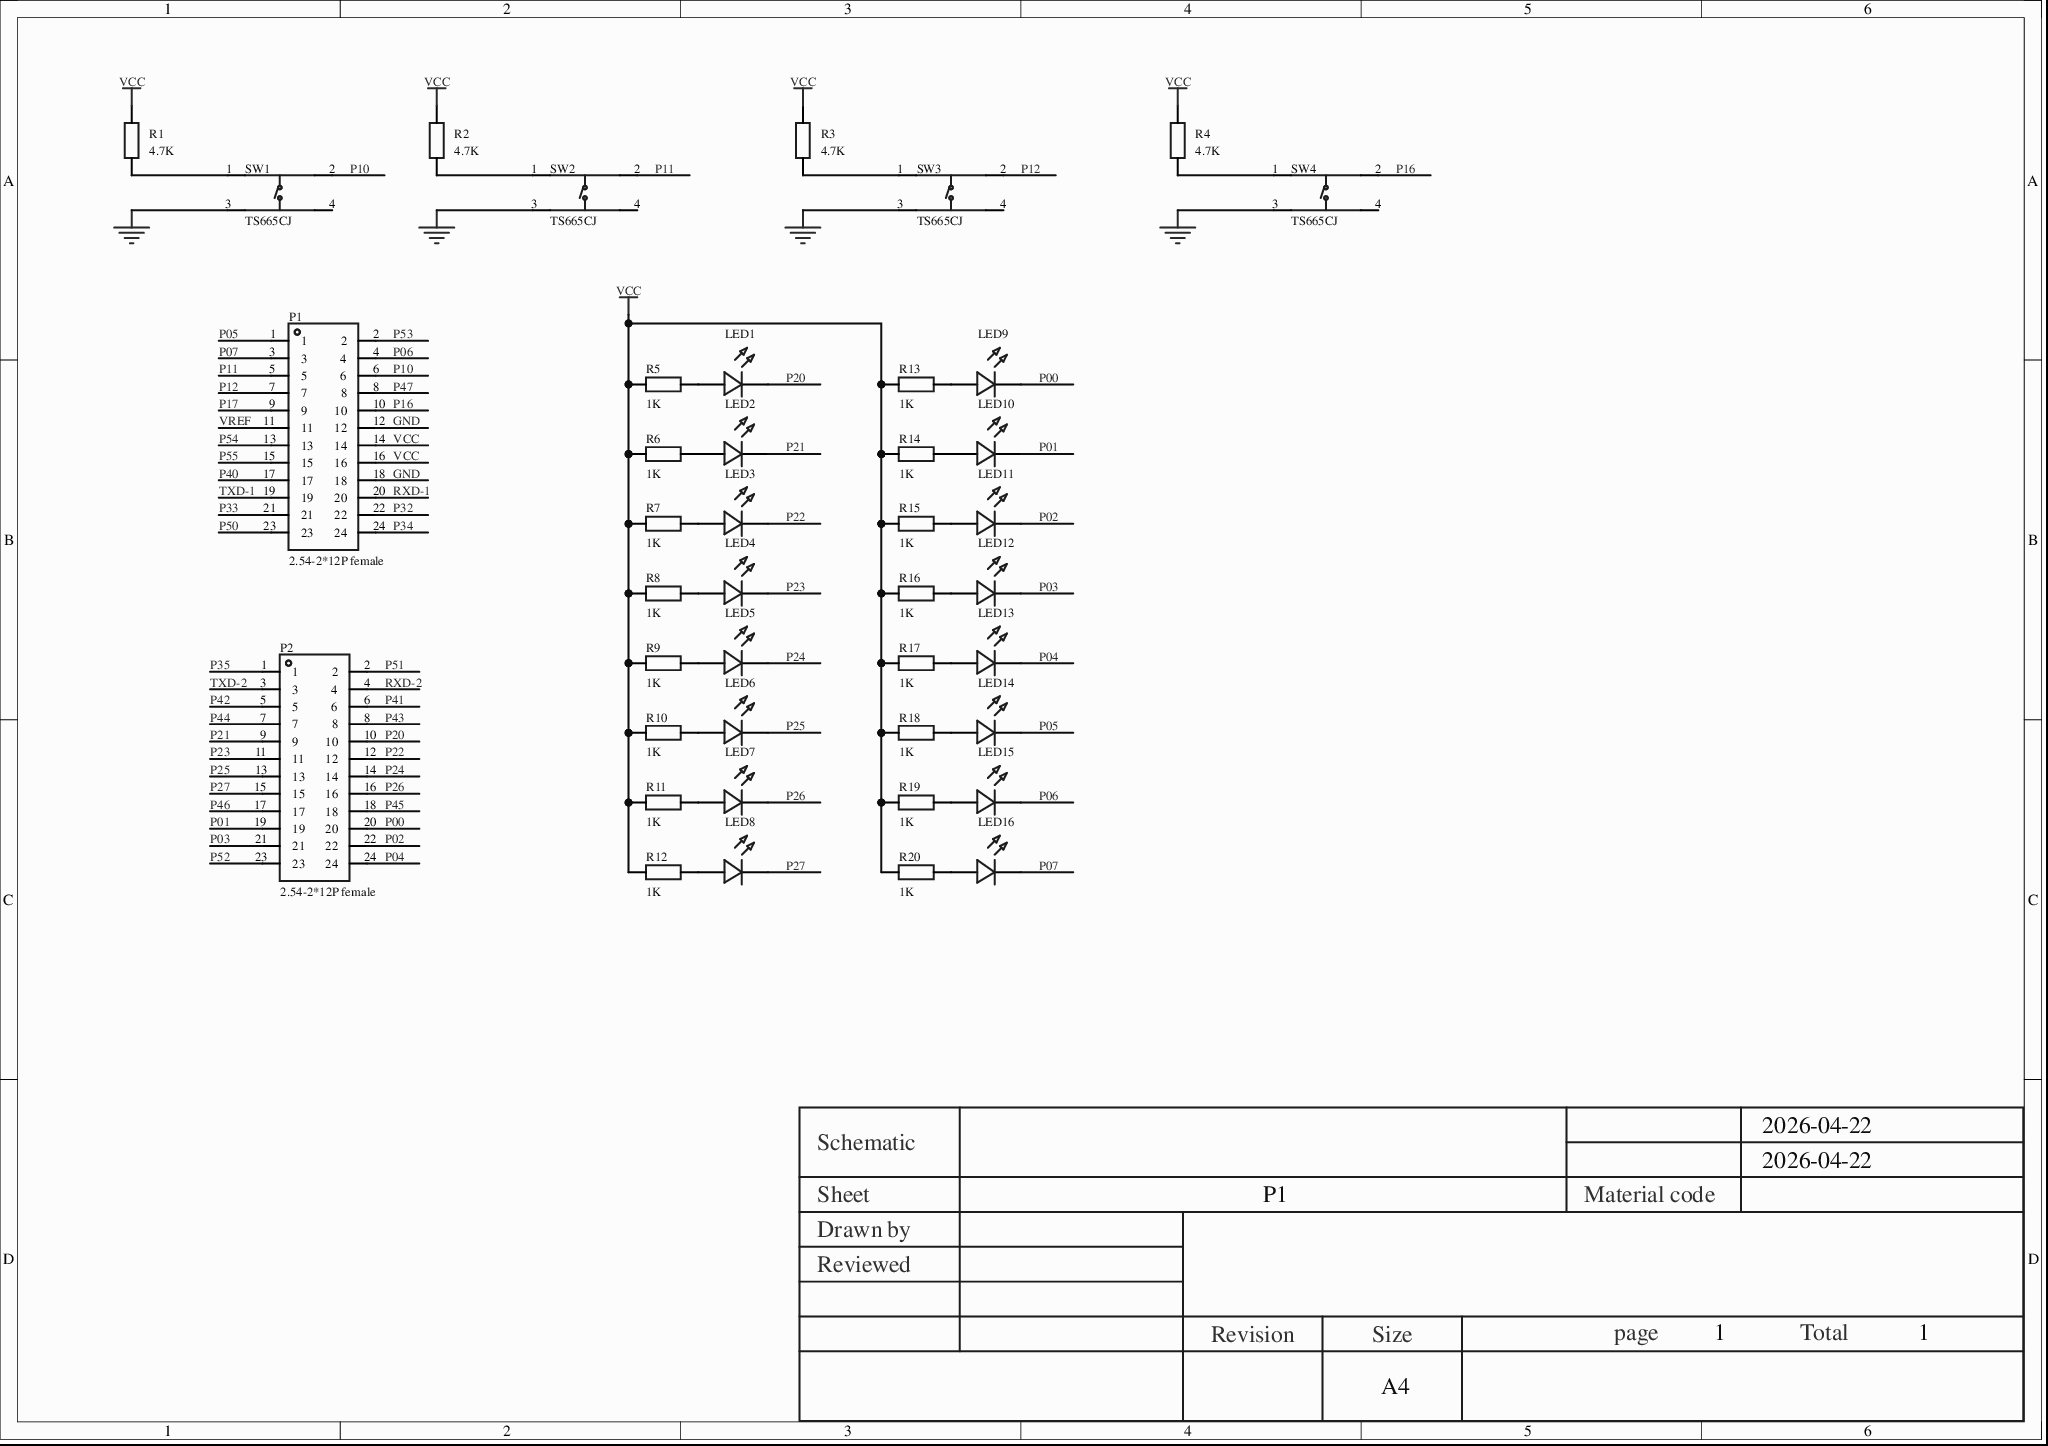
[diagram p0: MISC51818-3.schdoc]
# Altium project MISC51818-2.PrjPcb
1 sheet, 42 parts. Net scope: global (net labels, ports and power ports of the same name join across sheets).
Board file: MISC51818.pcbdoc

## Sheet MISC51818-3.schdoc
size 297 x 209 mm; Version: V1.0; @Project Name: MISC51818; @Page Count: 1; @Update Date: 2026-04-22; @Create Date: 2026-04-22; @Schematic Name: MISC51818; @Page No: 1; @Board Name: MISC51818; @Create Time: 22:35:28; @Update Time: 22:35:28

### Parts
LED1  (no value)  [LED-TH_L5.0-W5.0-P2.54_RED]
LED2  (no value)  [LED-TH_L5.0-W5.0-P2.54_RED]
LED3  (no value)  [LED-TH_L5.0-W5.0-P2.54_RED]
LED4  (no value)  [LED-TH_L5.0-W5.0-P2.54_RED]
LED5  (no value)  [LED-TH_L5.0-W5.0-P2.54_RED]
LED6  (no value)  [LED-TH_L5.0-W5.0-P2.54_RED]
LED7  (no value)  [LED-TH_L5.0-W5.0-P2.54_RED]
LED8  (no value)  [LED-TH_L5.0-W5.0-P2.54_RED]
LED9  (no value)  [LED-TH_L5.0-W5.0-P2.54_RED]
LED10  (no value)  [LED-TH_L5.0-W5.0-P2.54_RED]
LED11  (no value)  [LED-TH_L5.0-W5.0-P2.54_RED]
LED12  (no value)  [LED-TH_L5.0-W5.0-P2.54_RED]
LED13  (no value)  [LED-TH_L5.0-W5.0-P2.54_RED]
LED14  (no value)  [LED-TH_L5.0-W5.0-P2.54_RED]
LED15  (no value)  [LED-TH_L5.0-W5.0-P2.54_RED]
LED16  (no value)  [LED-TH_L5.0-W5.0-P2.54_RED]
P1  2.54-2*12P female  [HDR-TH_24P-P2.54-V-F-R2-C12-S2.54]
P2  2.54-2*12P female  [HDR-TH_24P-P2.54-V-F-R2-C12-S2.54]
R1  4.7K  [RES-TH_RES-TH_L6.5-W5.0-P2.50-D0.4-S2.00]
R2  4.7K  [RES-TH_RES-TH_L6.5-W5.0-P2.50-D0.4-S2.00]
R3  4.7K  [RES-TH_RES-TH_L6.5-W5.0-P2.50-D0.4-S2.00]
R4  4.7K  [RES-TH_RES-TH_L6.5-W5.0-P2.50-D0.4-S2.00]
R5  1K  [RES-TH_RES-TH_L6.5-W5.0-P2.50-D0.4-S2.00]
R6  1K  [RES-TH_RES-TH_L6.5-W5.0-P2.50-D0.4-S2.00]
R7  1K  [RES-TH_RES-TH_L6.5-W5.0-P2.50-D0.4-S2.00]
R8  1K  [RES-TH_RES-TH_L6.5-W5.0-P2.50-D0.4-S2.00]
R9  1K  [RES-TH_RES-TH_L6.5-W5.0-P2.50-D0.4-S2.00]
R10  1K  [RES-TH_RES-TH_L6.5-W5.0-P2.50-D0.4-S2.00]
R11  1K  [RES-TH_RES-TH_L6.5-W5.0-P2.50-D0.4-S2.00]
R12  1K  [RES-TH_RES-TH_L6.5-W5.0-P2.50-D0.4-S2.00]
R13  1K  [RES-TH_RES-TH_L6.5-W5.0-P2.50-D0.4-S2.00]
R14  1K  [RES-TH_RES-TH_L6.5-W5.0-P2.50-D0.4-S2.00]
R15  1K  [RES-TH_RES-TH_L6.5-W5.0-P2.50-D0.4-S2.00]
R16  1K  [RES-TH_RES-TH_L6.5-W5.0-P2.50-D0.4-S2.00]
R17  1K  [RES-TH_RES-TH_L6.5-W5.0-P2.50-D0.4-S2.00]
R18  1K  [RES-TH_RES-TH_L6.5-W5.0-P2.50-D0.4-S2.00]
R19  1K  [RES-TH_RES-TH_L6.5-W5.0-P2.50-D0.4-S2.00]
R20  1K  [RES-TH_RES-TH_L6.5-W5.0-P2.50-D0.4-S2.00]
SW1  TS665CJ  [SW-TH_4P-L6.0-W6.0-P4.50-LS6.5]
SW2  TS665CJ  [SW-TH_4P-L6.0-W6.0-P4.50-LS6.5]
SW3  TS665CJ  [SW-TH_4P-L6.0-W6.0-P4.50-LS6.5]
SW4  TS665CJ  [SW-TH_4P-L6.0-W6.0-P4.50-LS6.5]

### Nets
GND: P1.12 P1.18 SW1.3(C) SW2.3(C) SW3.3(C) SW4.3(C)
VCC: P1.14 P1.16 R1.2 R2.2 R3.2 R4.2 R5.1 R6.1 R7.1 R8.1 R9.1 R10.1 R11.1 R12.1 R13.1 R14.1 R15.1 R16.1 R17.1 R18.1 R19.1 R20.1
P00: LED9.1(C) P2.20
P01: LED10.1(C) P2.19
P02: LED11.1(C) P2.22
P03: LED12.1(C) P2.21
P04: LED13.1(C) P2.24
P05: LED14.1(C) P1.1
P06: LED15.1(C) P1.4
P07: LED16.1(C) P1.3
P10: P1.6 SW1.2(B)
P11: P1.5 SW2.2(B)
P12: P1.7 SW3.2(B)
P16: P1.10 SW4.2(B)
P17: P1.9
P20: LED1.1(C) P2.10
P21: LED2.1(C) P2.9
P22: LED3.1(C) P2.12
P23: LED4.1(C) P2.11
P24: LED5.1(C) P2.14
P25: LED6.1(C) P2.13
P26: LED7.1(C) P2.16
P27: LED8.1(C) P2.15
P32: P1.22
P33: P1.21
P34: P1.24
P35: P2.1
P40: P1.17
P41: P2.6
P42: P2.5
P43: P2.8
P44: P2.7
P45: P2.18
P46: P2.17
P47: P1.8
P50: P1.23
P51: P2.2
P52: P2.23
P53: P1.2
P54: P1.13
P55: P1.15
RXD-1: P1.20
RXD-2: P2.4
TXD-1: P1.19
TXD-2: P2.3
VREF: P1.11
NetLED1_2: LED1.2(A) R5.2
NetLED2_2: LED2.2(A) R6.2
NetLED3_2: LED3.2(A) R7.2
NetLED4_2: LED4.2(A) R8.2
NetLED5_2: LED5.2(A) R9.2
NetLED6_2: LED6.2(A) R10.2
NetLED7_2: LED7.2(A) R11.2
NetLED8_2: LED8.2(A) R12.2
NetLED9_2: LED9.2(A) R13.2
NetLED10_2: LED10.2(A) R14.2
NetLED11_2: LED11.2(A) R15.2
NetLED12_2: LED12.2(A) R16.2
NetLED13_2: LED13.2(A) R17.2
NetLED14_2: LED14.2(A) R18.2
NetLED15_2: LED15.2(A) R19.2
NetLED16_2: LED16.2(A) R20.2
NetR1_1: R1.1 SW1.1(A)
NetR2_1: R2.1 SW2.1(A)
NetR3_1: R3.1 SW3.1(A)
NetR4_1: R4.1 SW4.1(A)

Not connected (* = marked no-connect by the designer): SW1 4(D); SW2 4(D); SW3 4(D); SW4 4(D)

### Notes on the sheet
- 2026-04-22
- Schematic
- Sheet
- P1
- Material code
- Reviewed
- Drawn by
- Revision
- Size
- A4
- page
- 1
- Total

### Library data of the parts
LED1-LED16 = LED_0603-G: Symbol: LED_G; Convert to PCB: yes; 3D Model: 8b5fcaf0229049f8a37a9c352bb0ca0a0819f05c4eef4c71ace90d822a990e87; 3D Model Transform: 63.1,31.6,23.7,0,0,0,0,0,0; ModelName: LED-0603_G; Device: LED_0603-G; Add into BOM: yes; Supplier Footprint: 0603; FootprintName: LED-TH_L5.0-W5.0-P2.54_RED
P1 P2 = 2.54-2*12P母: Socket structure: 2x12P; pitch: 2.54mm; row spacing: 2.54mm; round/square hole: square hole; mounting: through-hole; rows: dual row; total positions: 24P; rated current: 3A; socket direction: top; plastic height: 2.5mm; contact material: brass; contact plating: -; operating temperature: -55℃~+105℃;; Manufacturer: BOOMELE(博穆精密); Symbol: Female header2*12PRight Angle/pitch2.54mm; AddInBom: yes; ModelId: 167707a4a3c342ff872f63f8f357b7a80819f05c4eef4c71ace90d822a990e87; ModelName: HDR-TH_24P-P2.54-F-LI-2X12P; ModelTransform: 1199.9976,200,0,0,0,0,0,0,-118.11; Device: 2.54-2*12P female; FootprintName: HDR-TH_24P-P2.54-V-F-R2-C12-S2.54; LCSC Part Name: 2x12P 间距:2.54mm 直插; SupplierPart: C62744; ManufacturerPart: 2.54-2*12P母; Supplier Footprint: 插件,P=2.54mm; JLCPCB Part Class: Extended Part; Datasheet: example.com/datasheet/2.54-2*12P%25E6%25AF%258D/63805.html; Supplier: LCSC; ConvertToPcb: yes; Holes Structure: 2x12P; Pitch: 2.54mm; Row Spacing: 2.54mm; Circular Hole / Square Hole: Square hole; Mounting Type: Through-hole; Number of Rows: Dual row; Number of Positions: 24P; Current Rating: 3A; Holes Direction: Top; Insulation Height: 2.5mm; Contact Material: Brass; Contact Plating: -; Operating Temperature: -55℃~+105℃
R1-R20 = Res_0603: Symbol: Resistor; ConvertToPcb: yes; ModelId: fc143cca1e79419f9cd78b61e9279f080819f05c4eef4c71ace90d822a990e87; ModelName: R0603; ModelTransform: 31.8897,63.7794,0,90,0,0,0,0,0; Device: Res_0603; FootprintName: RES-TH_RES-TH_L6.5-W5.0-P2.50-D0.4-S2.00; AddInBom: yes; Supplier Footprint: 0603
  R1-R4: Value: 4.7K
  R5-R20: Value: 1K
SW1-SW4 = TS665CJ: Circuit: SPST; button shape: round; actuating force: 2.5N; mounting: through-hole; length: 6mm; width: 6mm; height: 5mm; bracket: none; contact current: 50mA; rated voltage: 12V; lamp: none; life: 5 ten-thousand cycles;; Manufacturer: SHOU HAN(首韩); AddInBom: yes; Actuator Style: Round button; with Bracket: No bracket; Actuator/Cap Color: Black; ModelId: 20eee248bc684ccd8cbdbb1d0d91ec6f0819f05c4eef4c71ace90d822a990e87; ModelName: SW-TH_4P-L6.0-W6.0-H5.0-LS6.5-P4.50; ModelTransform: 236.22,323.03,0,90,0,0,0,0,-137.795; Device: TS665CJ; Symbol: TS665CJ; FootprintName: SW-TH_4P-L6.0-W6.0-P4.50-LS6.5; LCSC Part Name: 6*6*5mm 直插 轻触开关; SupplierPart: C393938; ManufacturerPart: TS665CJ; Supplier Footprint: 插件-4P,6x6mm; JLCPCB Part Class: Extended Part; Datasheet: example.com/datasheet/TS665CJ/372550.html; Supplier: LCSC; ConvertToPcb: yes; Operating Force: 2.5N; Mounting Type: Through-hole; Length: 6mm; Width: 6mm; Switch Height: 5mm; Contact Current: 50mA; Voltage Rating: 12V; With Lamp: None; Termination Style: PC pin; Life: 5 ten-thousand cycles; Operating Temperature: -25℃~+70℃